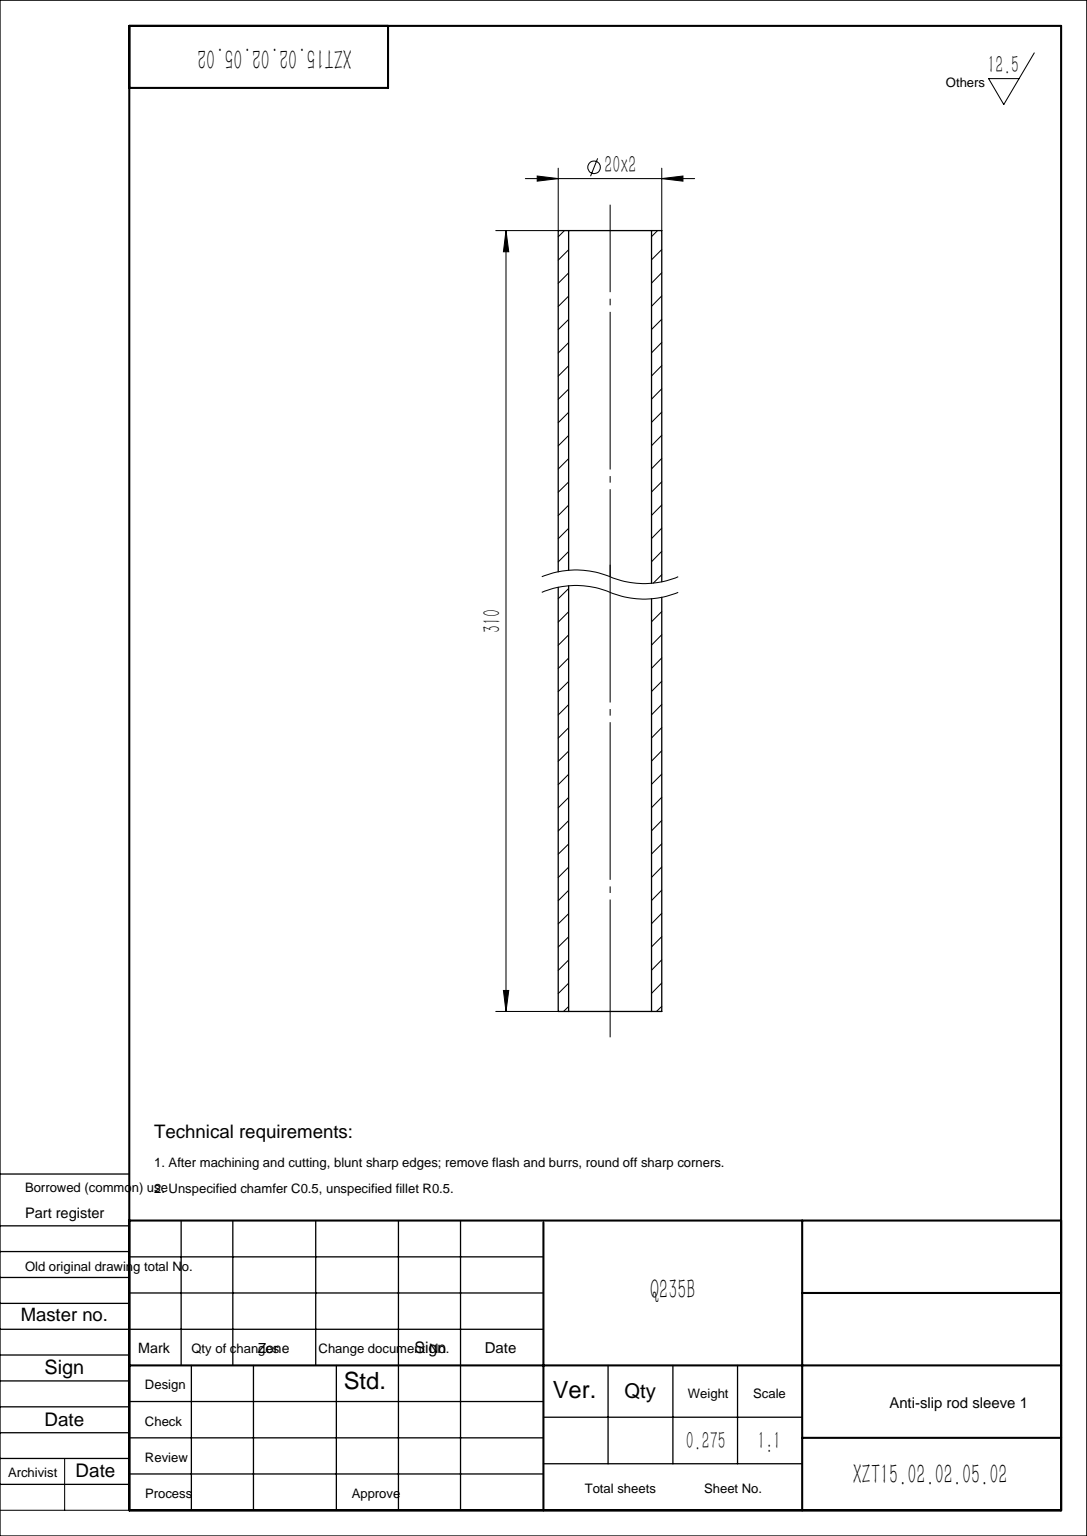
from build123d import *

# Parameters (mm, degrees)
SKETCH11_R                             = 10
SKETCH11_R_2                           = 8
GB_T_6728_2002_ROUND_TUBE_20_2_1_DEPTH = 310


with BuildPart() as part:
    # Sketch11 → Gb／t 6728—2002 round tube 20 × 2(1) (new body)
    with BuildSketch(Plane(origin=(0, 0, 0), x_dir=(-1, 0, 0), z_dir=(0, 1, 0))):
        Circle(SKETCH11_R)
        Circle(SKETCH11_R_2, mode=Mode.SUBTRACT)
    extrude(amount=GB_T_6728_2002_ROUND_TUBE_20_2_1_DEPTH)


solid = part.part
